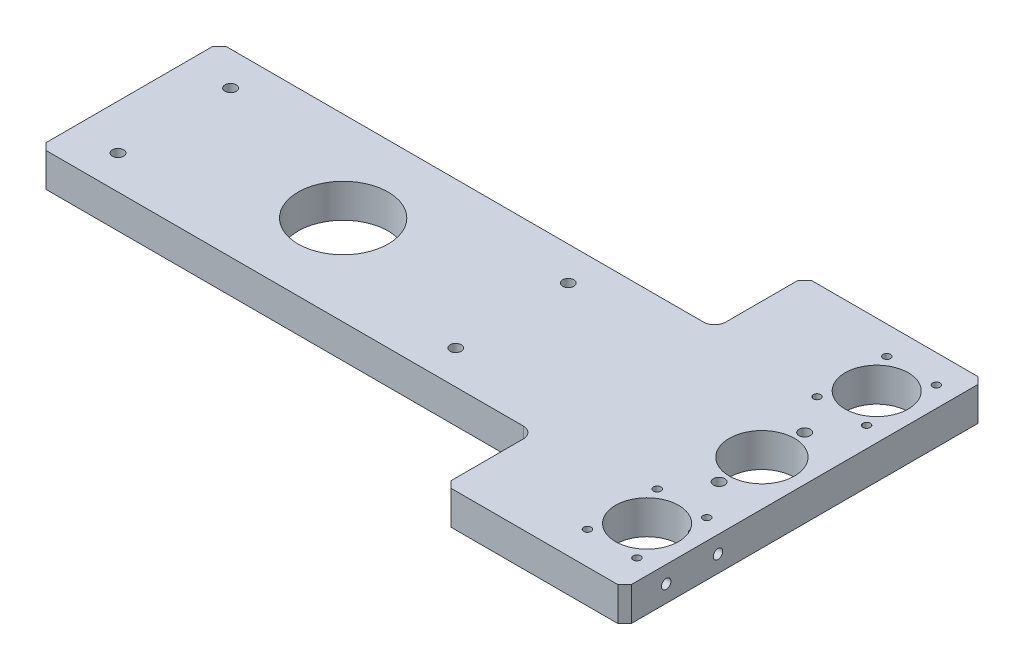
from build123d import *

# Parameters (mm, degrees)
SKETCH1_W             = 300
SKETCH1_H             = 160
BOSS_EXTRUDE1_DEPTH   = 15
CHAMFER1_SIZE         = 3
SKETCH2_R             = 14
CUT_EXTRUDE1_DEPTH    = 171.660481659
M4_TAPPED_HOLE1_D     = 3.3
SKETCH5_R             = 14.5
CUT_EXTRUDE2_DEPTH    = 171.660481659
M6_TAPPED_HOLE1_D     = 5
M5_TAPPED_HOLE2_D     = 4.2
M5_TAPPED_HOLE2_DEPTH = 14
M5_TAPPED_HOLE2_TIP   = 1.2618073
SKETCH17_W            = 220
SKETCH17_H            = 40
CUT_EXTRUDE6_DEPTH    = 171.660481755
M6_TAPPED_HOLE2_D     = 5
SKETCH20_R            = 20
CUT_EXTRUDE7_DEPTH    = 171.660481755
CHAMFER2_SIZE         = 3
FILLET1_R             = 5


with BuildPart() as part:
    # Sketch1 → Boss-Extrude1 (new body)
    with BuildSketch(Plane(origin=(0, 0, 0), x_dir=(1, 0, 0), z_dir=(0, 1, 0))):
        Rectangle(SKETCH1_W, SKETCH1_H)
    extrude(amount=BOSS_EXTRUDE1_DEPTH)

    # Chamfer1
    chamfer1_edges = [part.edges().sort_by_distance(p)[0] for p in [
        (-150, 7.5, -80),
        (150, 7.5, -80),
        (150, 7.5, 80),
        (-150, 7.5, 80),
    ]]
    chamfer(chamfer1_edges, length=CHAMFER1_SIZE)

    # Sketch2 → Cut-Extrude1 (cut, through all)
    with BuildSketch(Plane(origin=(0, 15, 0), x_dir=(1, 0, 0), z_dir=(0, 1, 0))):
        with Locations(Location((130, -50, 0), (0, 0, 270))):
            Circle(SKETCH2_R)
        with Locations(Location((130, 52, 0), (0, 0, 90))):
            Circle(SKETCH2_R)
    extrude(amount=-CUT_EXTRUDE1_DEPTH, mode=Mode.SUBTRACT)

    # M4 Tapped Hole1 (through all)
    with Locations(Plane(origin=(0, 15, 0), x_dir=(-1, 0, 0), z_dir=(0, 1, 0))):
        with Locations((-141, 34.5), (-119, -67.5), (-141, -67.5), (-119, -36.5), (-141, -36.5), (-119, 34.5), (-119, 65.5), (-141, 65.5)):
            Hole(M4_TAPPED_HOLE1_D / 2)

    # Sketch5 → Cut-Extrude2 (cut, through all)
    with BuildSketch(Plane(origin=(0, 15, 0), x_dir=(1, 0, 0), z_dir=(0, 1, 0))):
        with Locations(Location((130, 1, 0), (0, 0, 270))):
            Circle(SKETCH5_R)
    extrude(amount=-CUT_EXTRUDE2_DEPTH, mode=Mode.SUBTRACT)

    # M6 Tapped Hole1 (through all)
    with Locations(Plane(origin=(0, 15, 0), x_dir=(-1, 0, 0), z_dir=(0, 1, 0))):
        with Locations((-130, -20), (-130, 18)):
            Hole(M6_TAPPED_HOLE1_D / 2)

    # M5 Tapped Hole2
    with Locations(Plane(origin=(150, 0, 0), x_dir=(0, 0, -1), z_dir=(1, 0, 0))):
        with Locations((-38.5, 7.5), (-61.5, 7.5)):
            Hole(M5_TAPPED_HOLE2_D / 2, depth=M5_TAPPED_HOLE2_DEPTH)
            with Locations((0, 0, -(M5_TAPPED_HOLE2_DEPTH + M5_TAPPED_HOLE2_TIP / 2))):  # 118° drill point
                Cone(0, M5_TAPPED_HOLE2_D / 2, M5_TAPPED_HOLE2_TIP, mode=Mode.SUBTRACT)

    # Sketch17 → Cut-Extrude6 (cut, through all)
    with BuildSketch(Plane(origin=(0, 15, 0), x_dir=(1, 0, 0), z_dir=(0, 1, 0))):
        with Locations((-40, 60)):
            Rectangle(SKETCH17_W, SKETCH17_H)
        with Locations((-40, -60)):
            Rectangle(SKETCH17_W, SKETCH17_H)
    extrude(amount=-CUT_EXTRUDE6_DEPTH, mode=Mode.SUBTRACT)

    # M6 Tapped Hole2 (through all)
    with Locations(Plane(origin=(0, 15, 0), x_dir=(1, 0, 0), z_dir=(0, 1, 0))):
        with Locations((-130, 25), (-130, -25), (20, -25), (20, 25)):
            Hole(M6_TAPPED_HOLE2_D / 2)

    # Sketch20 → Cut-Extrude7 (cut, through all)
    with BuildSketch(Plane(origin=(0, 15, 0), x_dir=(1, 0, 0), z_dir=(0, 1, 0))):
        with Locations(Location((-55, 0, 0), (0, 0, 270))):
            Circle(SKETCH20_R)
    extrude(amount=-CUT_EXTRUDE7_DEPTH, mode=Mode.SUBTRACT)

    # Chamfer2
    chamfer2_edges = [part.edges().sort_by_distance(p)[0] for p in [
        (70, 7.5, -80),
        (-150, 7.5, -40),
        (-150, 7.5, 40),
        (70, 7.5, 80),
    ]]
    chamfer(chamfer2_edges, length=CHAMFER2_SIZE)

    # Fillet1
    fillet1_edges = [part.edges().sort_by_distance(p)[0] for p in [
        (70, 7.5, -40),
        (70, 7.5, 40),
    ]]
    fillet(fillet1_edges, radius=FILLET1_R)


solid = part.part
